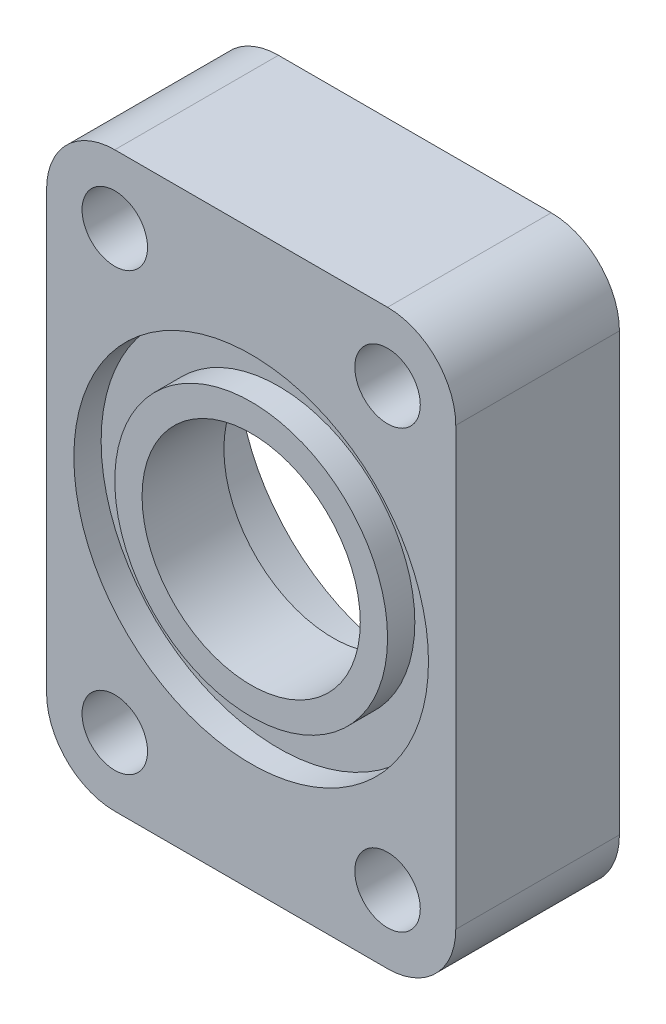
SolidWorks part; units mm, degrees
ref_plane "Front Plane" through (0, 0, 0) normal (0, 0, 1) x (1, 0, 0)
ref_plane "Top Plane" through (0, 0, 0) normal (0, 1, 0) x (1, 0, 0)
ref_plane "Right Plane" through (0, 0, 0) normal (1, 0, 0) x (0, 0, -1)
sketch "Sketch1" plane through (0, 0, 0) normal (0, 0, 1) x (1, 0, 0)
  line L1 (7.5, 0) -> (7.5, 7.5)
  line L2 (7.5, 7.5) -> (-7.5, 7.5)
  line L3 (-7.5, 7.5) -> (-7.5, -7.5)
  line L4 (-7.5, -7.5) -> (7.5, -7.5)
  line L5 (7.5, -7.5) -> (7.5, 0)
  circle A0 centre (0, 0) radius 4
extrude "Boss-Extrude1" add sketch "Sketch1" along normal blind 6
sketch "Sketch3" plane through (0, 0, 0) normal (0, 0, -1) x (-1, 0, 0)
  circle A0 centre (0, 0) radius 6.5
extrude "Cut-Extrude2" cut sketch "Sketch3" against normal blind 3
sketch "Sketch4" plane through (0, 0, 6) normal (0, 0, 1) x (1, 0, 0)
  circle A0 centre (0, 0) radius 5
  circle A1 centre (0, 0) radius 6.5
extrude "Cut-Extrude3" cut sketch "Sketch4" against normal blind 1
sketch "Sketch5" plane through (0, 0, 0) normal (0, 0, -1) x (-1, 0, 0)
  line L1 (7.5, -7.5) -> (-7.5, -7.5)
  line L2 (7.5, -7.5) -> (7.5, -10.5)
  line L3 (7.5, -10.5) -> (-7.5, -10.5)
  line L4 (-7.5, -7.5) -> (-7.5, -10.5)
  line L5 (-7.5, 7.5) -> (7.5, 7.5)
  line L6 (-7.5, 7.5) -> (-7.5, 10.5)
  line L7 (-7.5, 10.5) -> (7.5, 10.5)
  line L8 (7.5, 7.5) -> (7.5, 10.5)
extrude "Boss-Extrude2" add sketch "Sketch5" against normal blind 6
sketch "Sketch6" plane through (0, 0, 0) normal (0, 0, -1) x (-1, 0, 0)
  line L1 (7.5, 10.5) -> (7.5, -10.5) construction
  line L2 (7.5, 10.5) -> (-7.5, 10.5) construction
  circle A0 centre (5, 8) radius 1.2
  circle A1 centre (5, 8) radius 2.2 construction
  circle A2 centre (-5, 8) radius 1.2
  circle A3 centre (-5, -8) radius 1.2
  circle A4 centre (5, -8) radius 1.2
  dimension "D1" = 2.5
  dimension "D2" = 2.5
  dimension "D3" = 2
  dimension "D4" = 2
extrude "Cut-Extrude7" cut sketch "Sketch6" against normal blind 17
fillet "Fillet3" radius 2.5 4 edges at (-7.5, 10.5, 3) (-7.5, -10.5, 3) (7.5, -10.5, 3) (7.5, 10.5, 3)
sketch "Sketch7" plane through (0, 0, 0) normal (0, 0, -1) x (-1, 0, 0)
  circle A0 centre (-5, -8) radius 2.2
  circle A1 centre (-5, 8) radius 2.2
  circle A2 centre (5, 8) radius 2.2
  circle A3 centre (5, -8) radius 2.2
extrude "Cut-Extrude8" cut sketch "Sketch7" against normal blind 4
